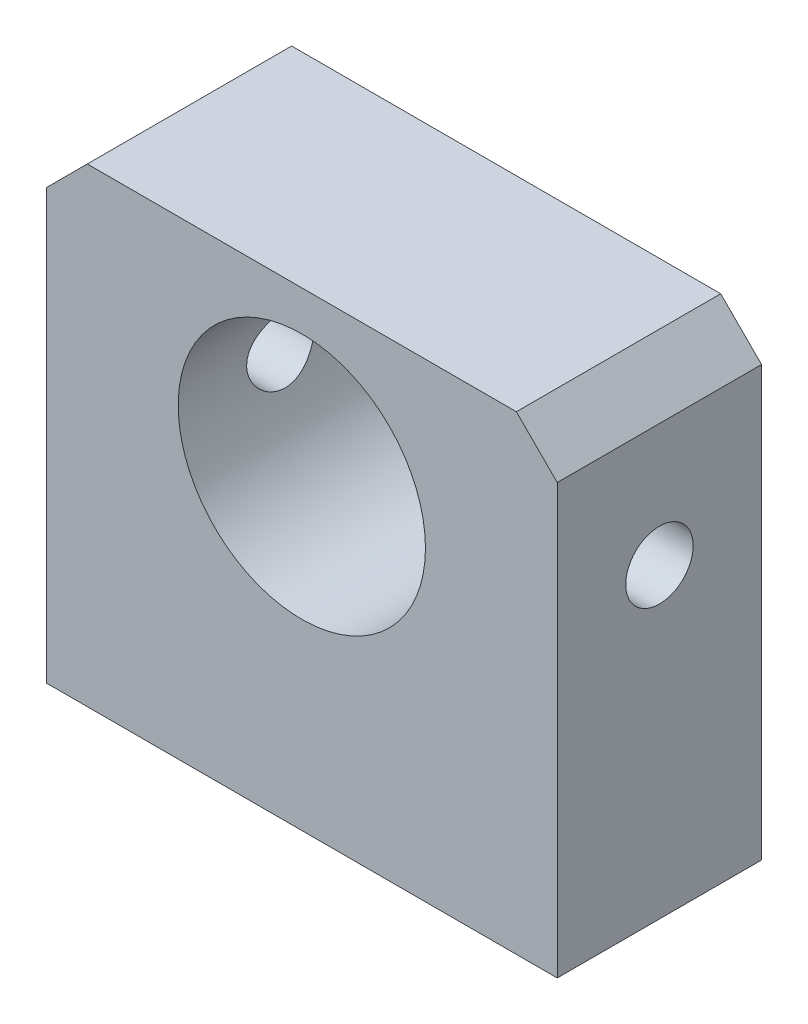
SolidWorks part; units mm, degrees
ref_plane "Front Plane" through (0, 0, 0) normal (0, 0, 1) x (1, 0, 0)
ref_plane "Top Plane" through (0, 0, 0) normal (0, 1, 0) x (1, 0, 0)
ref_plane "Right Plane" through (0, 0, 0) normal (1, 0, 0) x (0, 0, -1)
sketch "Sketch1" plane through (0, 0, 0) normal (0, 0, 1) x (1, 0, 0)
  line L1 (-12.5, -11.5) -> (12.5, -11.5)
  line L2 (-12.5, -11.5) -> (-12.5, 11.5)
  line L3 (-12.5, 11.5) -> (12.5, 11.5)
  line L4 (12.5, -11.5) -> (12.5, 11.5)
  line L5 (-12.5, -11.5) -> (12.5, 11.5) construction
  line L6 (-12.5, 11.5) -> (12.5, -11.5) construction
  point P0 (0, 0)
  dimension "D1" = 25
  dimension "D2" = 23
extrude "Boss-Extrude1" add sketch "Sketch1" along normal blind 10
sketch "Sketch2" plane through (0, 0, 10) normal (0, 0, 1) x (1, 0, 0)
  line L0 (12.5, 11.5) -> (-12.5, 11.5) construction
  circle A0 centre (0, 3.5) radius 6.05
  dimension "D1" = 12.1
  dimension "D2" = 8
extrude "Cut-Extrude1" cut sketch "Sketch2" against normal through all
chamfer "Chamfer1" distance 2 angle 45 2 edges at (12.5, 11.5, 5) (-12.5, 11.5, 5)
hole_wizard "M4 Tapped Hole1" positions "Sketch4" profile "Sketch3" tap size "M4" standard "GB"
sketch "Sketch4" plane through (0, -11.5, 0) normal (0, -1, 0) x (1, 0, 0)
  line L0 (0, 0) -> (0, 10) construction
  line L1 (-12.5, 10) -> (12.5, 10) construction
  line L3 (-12.5, 5) -> (12.5, 5) construction
  line L4 (-12.5, 10) -> (-12.5, 0) construction
  line L5 (12.5, 10) -> (12.5, 0) construction
  point P1 (-7, 5)
  point P3 (7, 5)
  dimension "D1" = 14
sketch "Sketch3" plane through (-7, -11.5, 5) normal (1, 0, 0) x (0, 0, -1)
  line L0 (0, 0) -> (0, 11.0914)
  line L1 (0, 11.0914) -> (1.65, 10.1)
  line L2 (1.65, 10.1) -> (1.65, 0)
  line L5 (1.65, 0) -> (0, 0)
  line L10 (0, 11.0914) -> (-1.65, 10.1) construction
  line L11 (0, -6.35) -> (0, 107.95) construction
  dimension "螺纹孔钻头直径" = 3.3
  dimension "螺纹孔钻头深度" = 10.1
  dimension "导头角度" = 118
cosmetic thread "Cosmetic Thread1" parameters "D1"=8, "D2"=4
cosmetic thread "Cosmetic Thread2" parameters "D1"=8, "D2"=4
hole_wizard "M4 Tapped Hole2" positions "Sketch6" profile "Sketch5" tap size "M4" standard "GB"
sketch "Sketch6" plane through (-12.5, 0, 0) normal (-1, 0, 0) x (0, 0, 1)
  line L0 (10, 9.5) -> (10, -11.5) construction
  line L1 (10, -11.5) -> (0, -11.5) construction
  point P0 (5, 3.5)
  dimension "D1" = 5
  dimension "D2" = 15
sketch "Sketch5" plane through (-12.5, 3.5, 5) normal (0, 1, 0) x (0, 0, 1)
  line L0 (0, 0) -> (0, 11.0914)
  line L1 (0, 11.0914) -> (1.65, 10.1)
  line L2 (1.65, 10.1) -> (1.65, 0)
  line L5 (1.65, 0) -> (0, 0)
  line L10 (0, 11.0914) -> (-1.65, 10.1) construction
  line L11 (0, -6.35) -> (0, 107.95) construction
  dimension "螺纹孔钻头直径" = 3.3
  dimension "螺纹孔钻头深度" = 10.1
  dimension "导头角度" = 118
cosmetic thread "Cosmetic Thread3" parameters "D1"=6.3164, "D2"=4
mirror "Mirror1" about plane through (0, 0, 0) normal (1, 0, 0) of "M4 Tapped Hole2"
